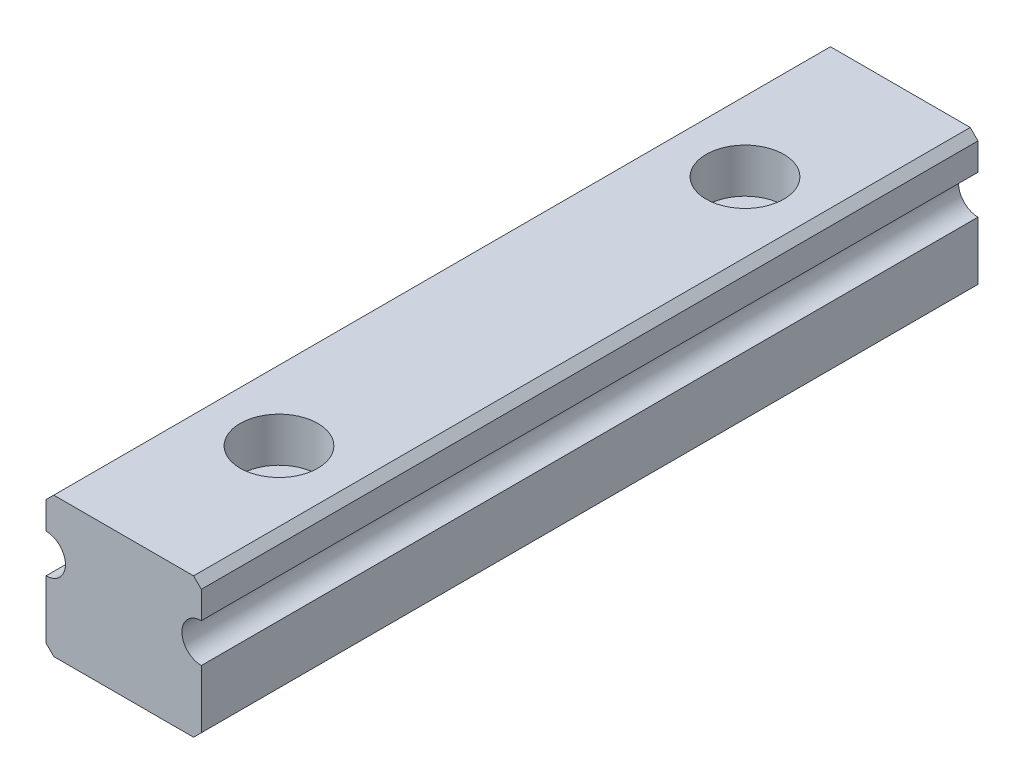
from build123d import *

# Parameters (mm, degrees)
EXTRUDE1_DEPTH                                       = 100
HOLE_SIZE_PER_SOCKET_HEAD_CAP_SCREW_TYPE_D           = 5.5
HOLE_SIZE_PER_SOCKET_HEAD_CAP_SCREW_TYPE_CBORE_D     = 10
HOLE_SIZE_PER_SOCKET_HEAD_CAP_SCREW_TYPE_CBORE_DEPTH = 5.7


with BuildPart() as part:
    # Sketch1 → Extrude1 (new body)
    with BuildSketch(Plane.XY):
        with BuildLine():
            Line((0, 13.5), (0, 17))
            Line((0, 17), (1, 18))
            Line((1, 18), (19, 18))
            Line((19, 18), (20, 17))
            Line((20, 17), (20, 13.5))
            ThreePointArc((20, 13.5), (17.5, 11), (20, 8.5))
            Line((20, 8.5), (20, 1))
            Line((20, 1), (19, 0))
            Line((19, 0), (1, 0))
            Line((1, 0), (0, 1))
            Line((0, 1), (0, 8.5))
            ThreePointArc((0, 8.5), (2.5, 11), (0, 13.5))
        make_face()
    extrude(amount=EXTRUDE1_DEPTH)

    # Hole size per socket head cap screw type 1 (through all)
    with Locations(Plane(origin=(10, 18, 20), x_dir=(0, 0, 1), z_dir=(0, 1, 0))):
        with Locations((0, 0), (60, 0)):
            CounterBoreHole(HOLE_SIZE_PER_SOCKET_HEAD_CAP_SCREW_TYPE_D / 2, HOLE_SIZE_PER_SOCKET_HEAD_CAP_SCREW_TYPE_CBORE_D / 2, HOLE_SIZE_PER_SOCKET_HEAD_CAP_SCREW_TYPE_CBORE_DEPTH)


solid = part.part
